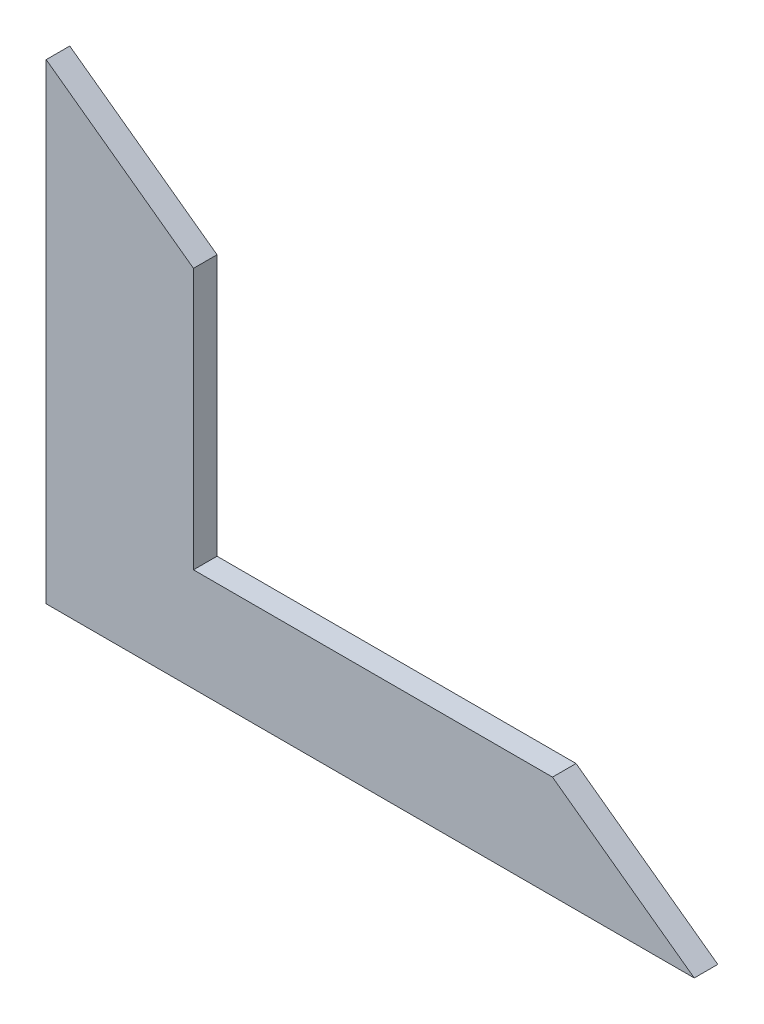
from build123d import *

# Parameters (mm, degrees)
EXTRUDE_1_DEPTH        = 8
HOLE_WIZARD_M4_1_D     = 3.3
HOLE_WIZARD_M4_1_DEPTH = 15
HOLE_WIZARD_M4_1_TIP   = 0.991420021
HOLE_WIZARD_M4_2_D     = 3.3
HOLE_WIZARD_M4_2_DEPTH = 15.1
HOLE_WIZARD_M4_2_TIP   = 0.991420021


with BuildPart() as part:
    # 草图1 → 凸台-拉伸1 (new body)
    with BuildSketch(Plane.XY):
        Polygon((-140, 40), (-140, -120), (80, -120), (31.875, -85), (-90, -85), (-90, 3.636363636), align=None)
    extrude(amount=EXTRUDE_1_DEPTH)

    # M4 螺纹孔1
    with Locations(Plane(origin=(0, -120, 0), x_dir=(-1, 0, 0), z_dir=(0, -1, 0))):
        with Locations((112.5, -4), (57.5, -4), (2.5, -4), (-52.5, -4)):
            Hole(HOLE_WIZARD_M4_1_D / 2, depth=HOLE_WIZARD_M4_1_DEPTH)
            with Locations((0, 0, -(HOLE_WIZARD_M4_1_DEPTH + HOLE_WIZARD_M4_1_TIP / 2))):  # 118° drill point
                Cone(0, HOLE_WIZARD_M4_1_D / 2, HOLE_WIZARD_M4_1_TIP, mode=Mode.SUBTRACT)

    # M4 螺纹孔2
    with Locations(Plane.ZY.offset(140)):
        with Locations((4, 20), (4, -40), (4, -100)):
            Hole(HOLE_WIZARD_M4_2_D / 2, depth=HOLE_WIZARD_M4_2_DEPTH)
            with Locations((0, 0, -(HOLE_WIZARD_M4_2_DEPTH + HOLE_WIZARD_M4_2_TIP / 2))):  # 118° drill point
                Cone(0, HOLE_WIZARD_M4_2_D / 2, HOLE_WIZARD_M4_2_TIP, mode=Mode.SUBTRACT)


solid = part.part
